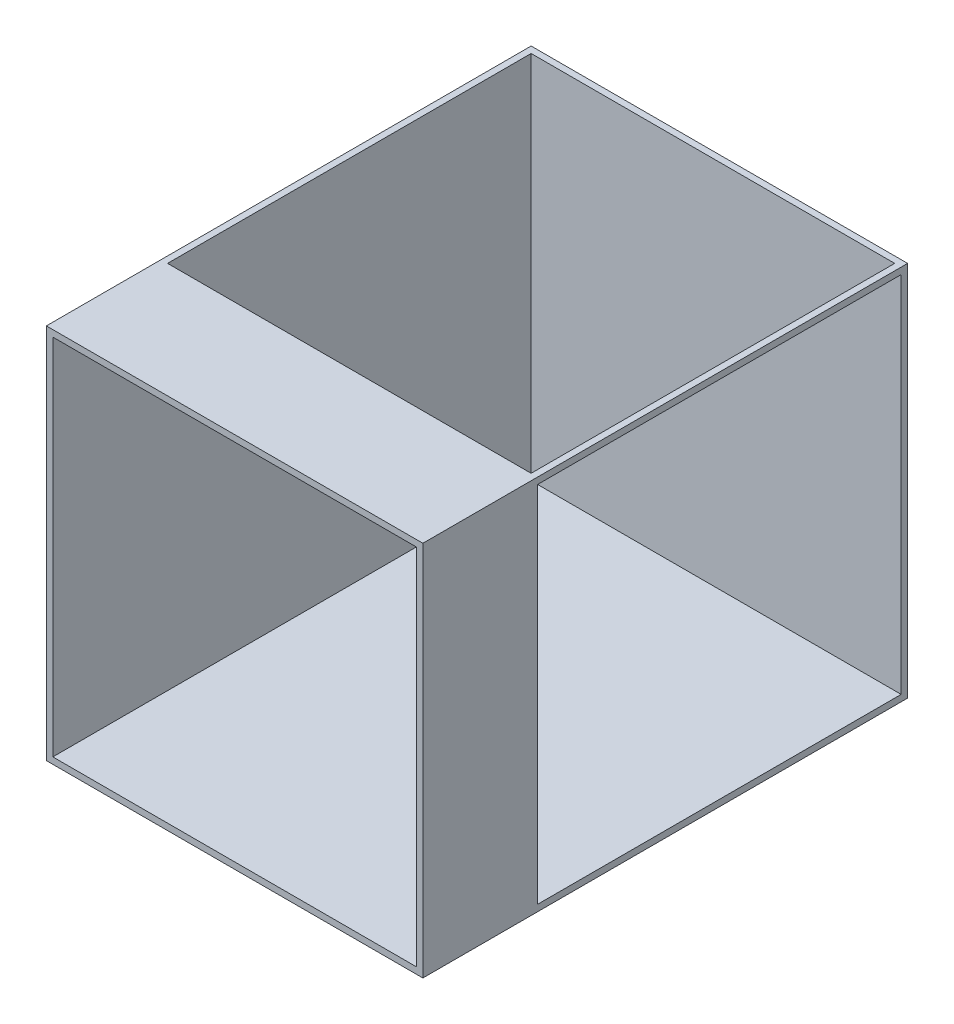
from build123d import *

# Parameters (mm, degrees)
SKETCH2_W           = 466
SKETCH2_H           = 466
SKETCH2_W_2         = 450
SKETCH2_H_2         = 450
BOSS_EXTRUDE1_DEPTH = 300
SKETCH4_W           = 8
SKETCH4_H           = 466
BOSS_EXTRUDE2_DEPTH = 450
SKETCH5_W           = 450
SKETCH5_H           = 450
CUT_EXTRUDE1_DEPTH  = 8
SKETCH6_W           = 450
SKETCH6_H           = 450
CUT_EXTRUDE2_DEPTH  = 8


with BuildPart() as part:
    # Sketch2 → Boss-Extrude1 (new, symmetric)
    with BuildSketch(Plane.XY):
        Rectangle(SKETCH2_W, SKETCH2_H)
        Rectangle(SKETCH2_W_2, SKETCH2_H_2, mode=Mode.SUBTRACT)
    extrude(amount=BOSS_EXTRUDE1_DEPTH, both=True)

    # Sketch4 → Boss-Extrude2 (add)
    with BuildSketch(Plane(origin=(-225, 0, 0), x_dir=(0, 0, -1), z_dir=(1, 0, 0))):
        with Locations((296, 0)):
            Rectangle(SKETCH4_W, SKETCH4_H)
    extrude(amount=BOSS_EXTRUDE2_DEPTH)

    # Sketch5 → Cut-Extrude1 (cut)
    with BuildSketch(Plane(origin=(0, 233, 0), x_dir=(1, 0, 0), z_dir=(0, 1, 0))):
        with Locations((0, 67)):
            Rectangle(SKETCH5_W, SKETCH5_H)
    extrude(amount=-CUT_EXTRUDE1_DEPTH, mode=Mode.SUBTRACT)

    # Sketch6 → Cut-Extrude2 (cut)
    with BuildSketch(Plane(origin=(233, 0, 0), x_dir=(0, 0, -1), z_dir=(1, 0, 0))):
        with Locations((67, 0)):
            Rectangle(SKETCH6_W, SKETCH6_H)
    extrude(amount=-CUT_EXTRUDE2_DEPTH, mode=Mode.SUBTRACT)


solid = part.part
